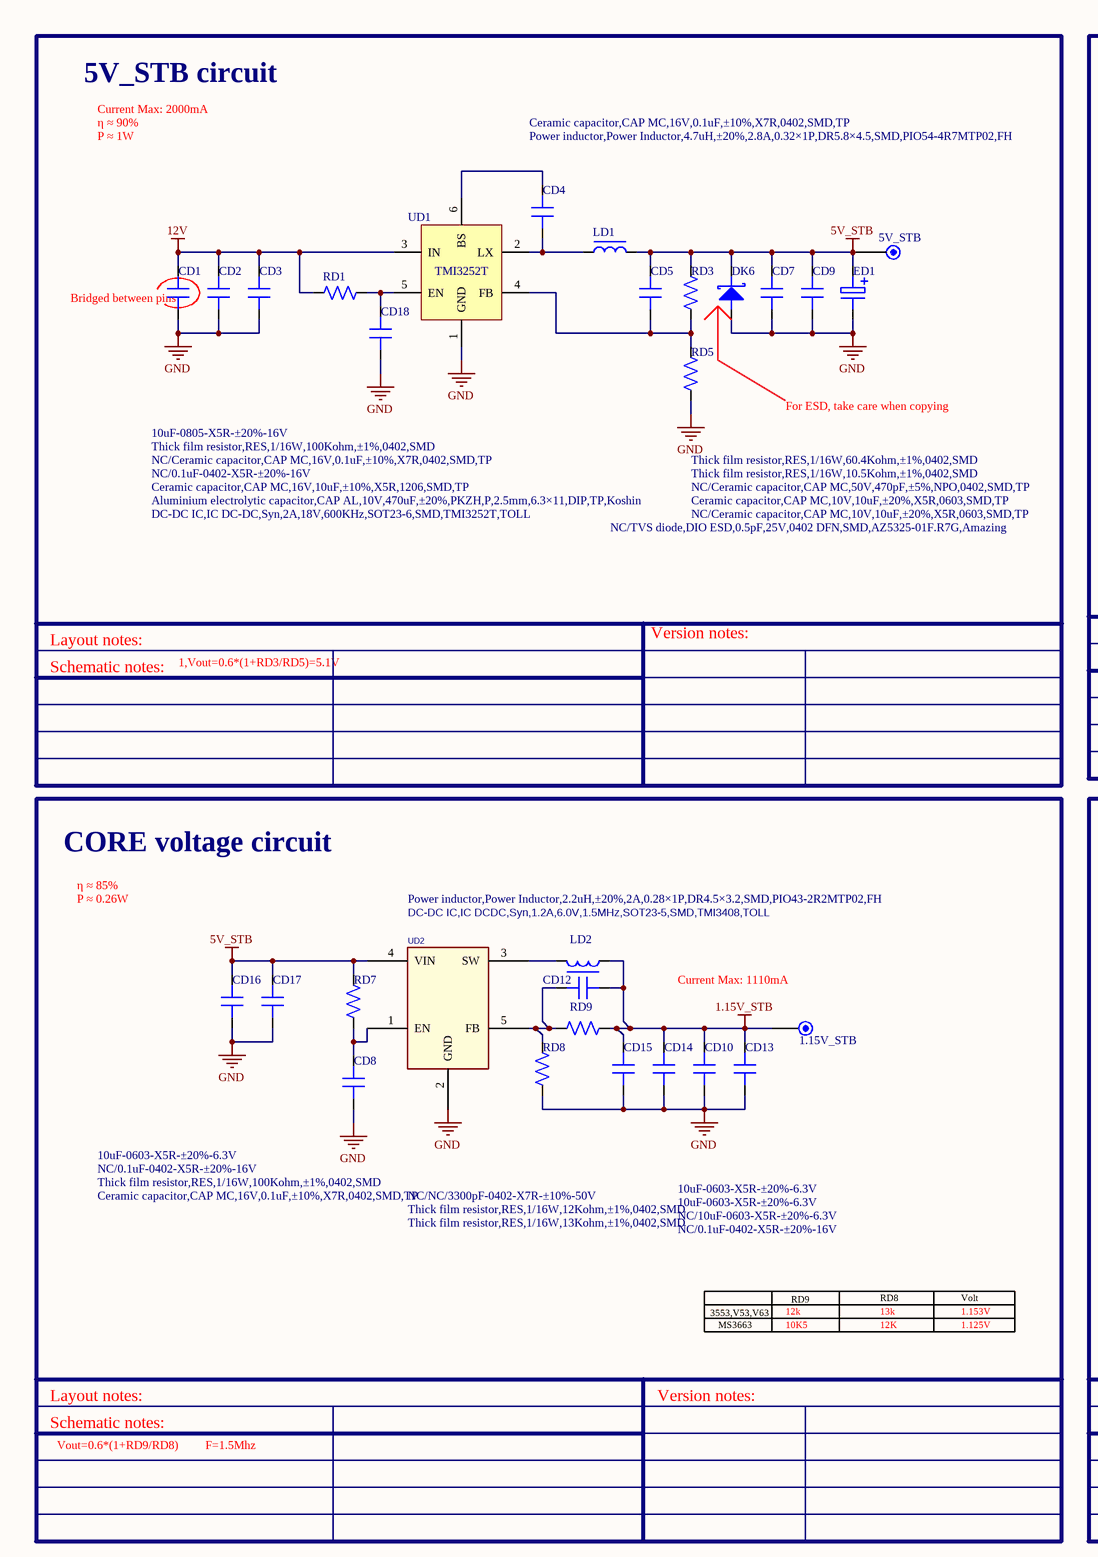
[diagram p0: MISC86383-11.SchDoc, left]
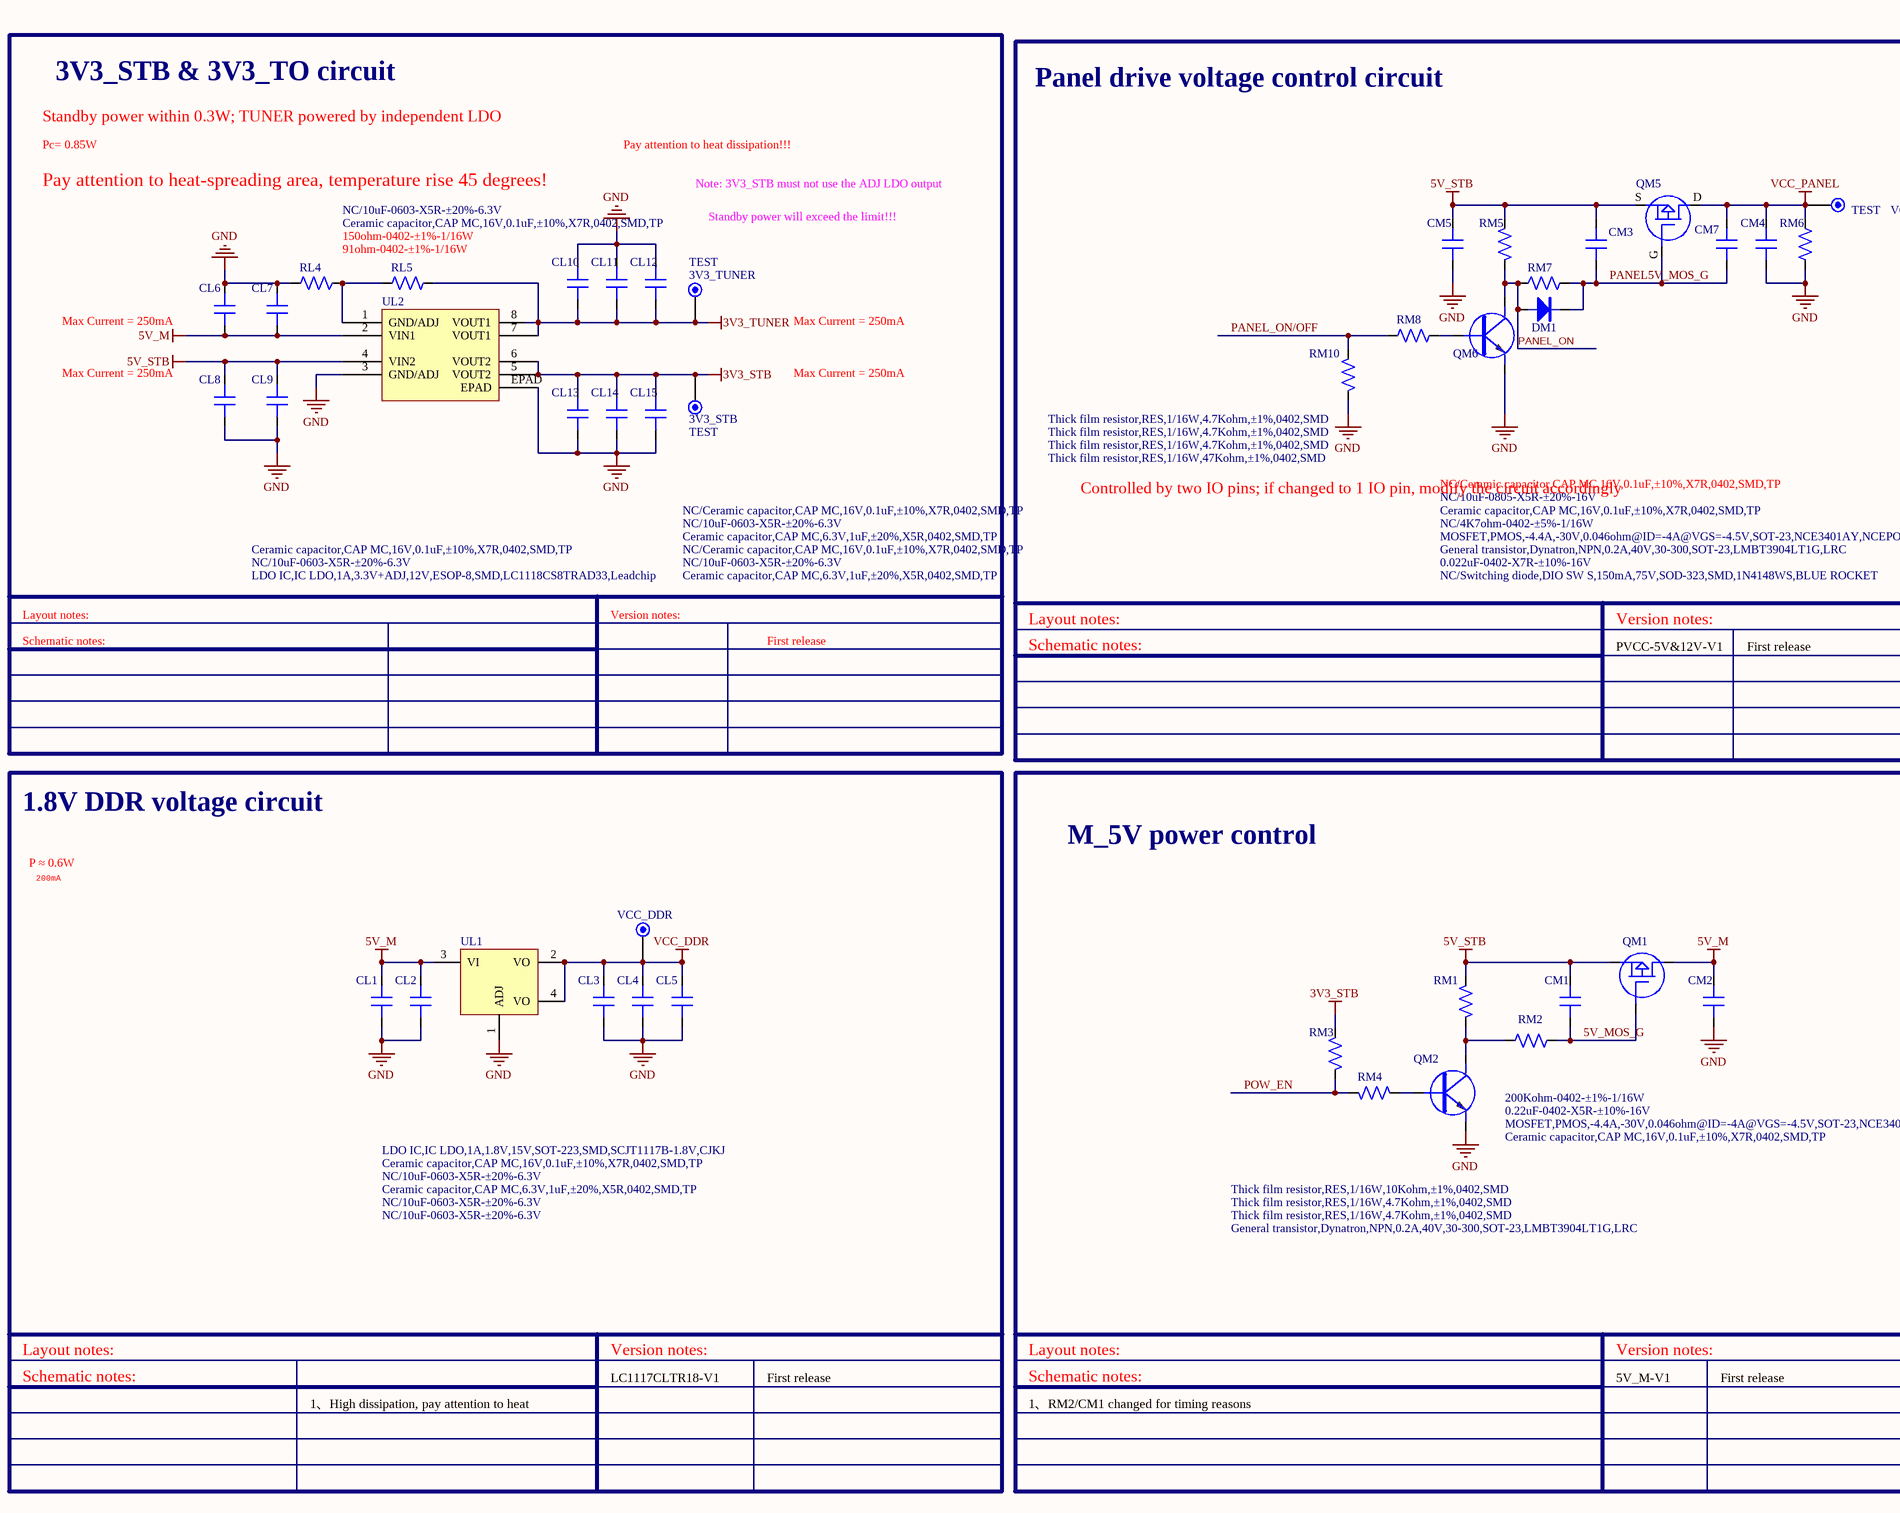
[diagram p1: MISC86383-11.SchDoc, middle]
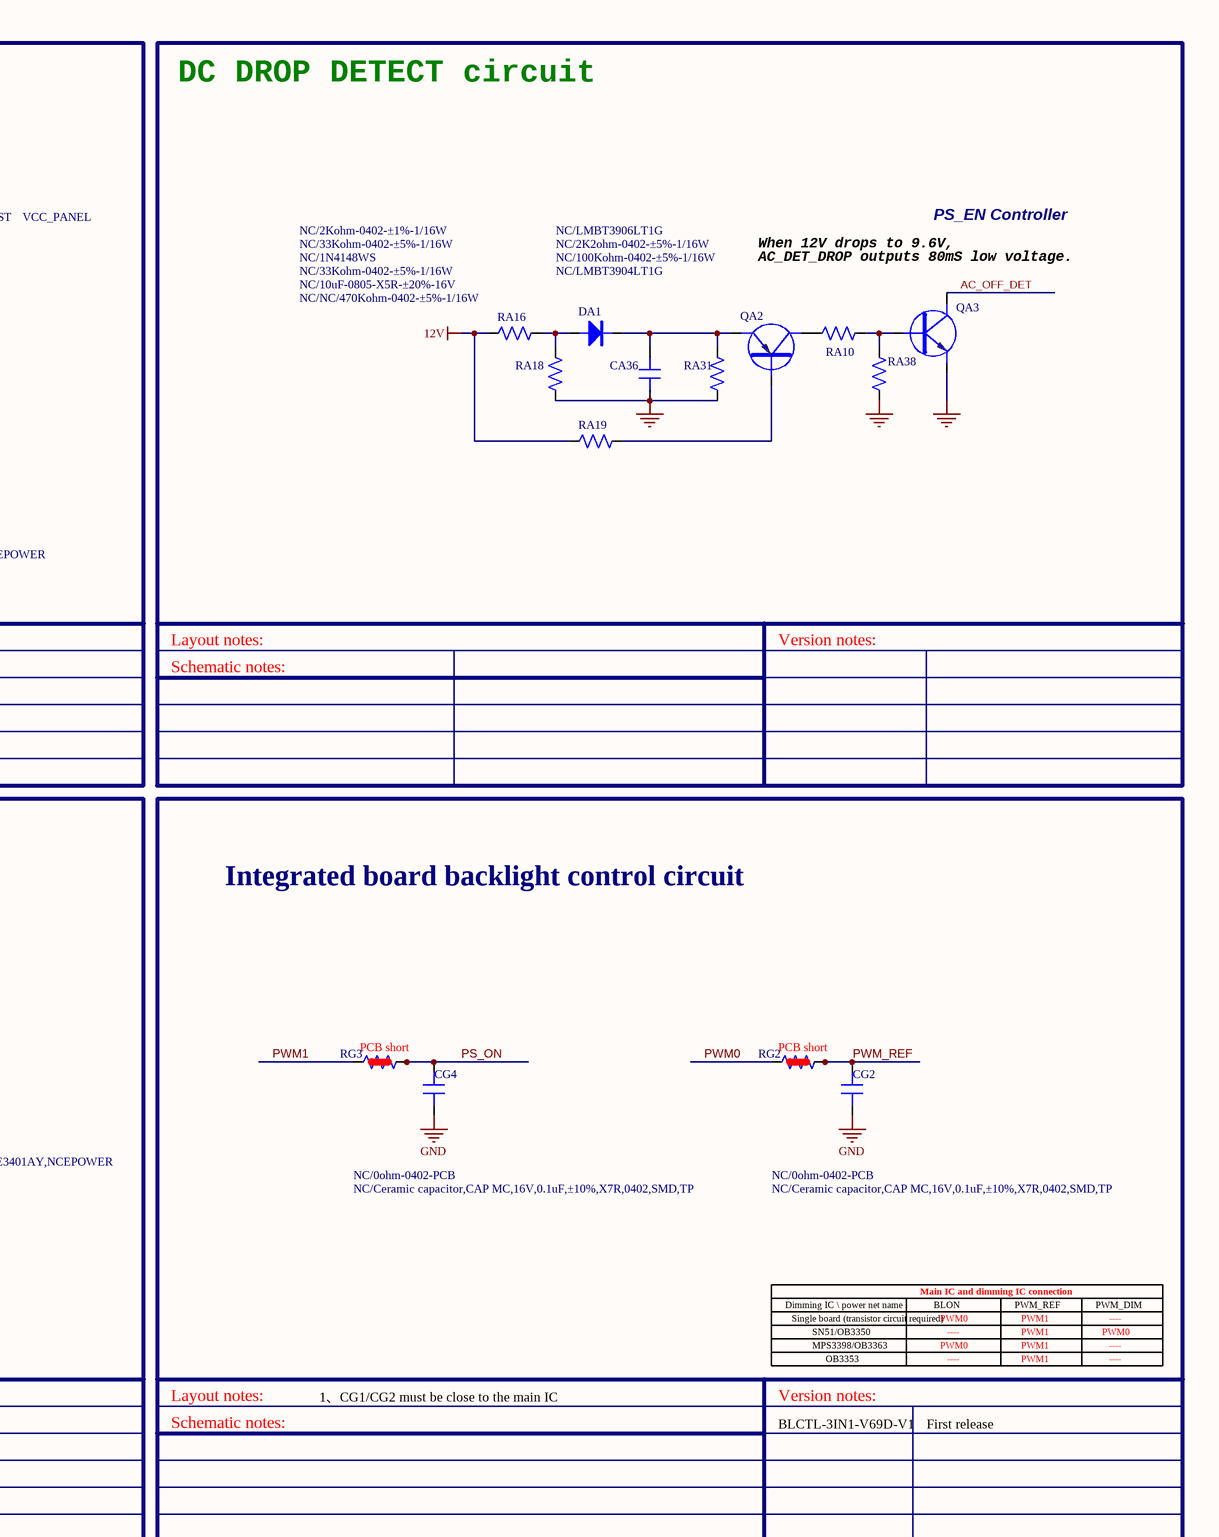
[diagram p2: MISC86383-11.SchDoc, right]
# Altium project MISC86383-33.PrjPCB (part 1 of 8)
9 sheets, 719 parts. Net scope: global (net labels, ports and power ports of the same name join across sheets).
Board files: MISC86383-7.PcbDoc, MISC86383.PcbDoc, MISC86383-9.PcbDoc
Sheets:
  MISC86383-11.SchDoc
  MISC86383-12.SchDoc
  MISC86383-13.SchDoc
  MISC86383-14.SchDoc
  MISC86383-15.SchDoc
  MISC86383-16.SchDoc
  MISC86383-18.SchDoc
  MISC86383-19.SchDoc
  MISC86383-5.SchDoc

## Sheet MISC86383-11.SchDoc
size 812 x 317 mm

### Parts
1.15V_STB  TEST  [TP]  (value not drawn)
3V3_STB  TEST  [TP]
3V3_TUNER  TEST  [TP]
5V_STB  TEST  [TP]  (value not drawn)
CA36  NC/10uF-0805-X5R-±20%-16V  [C0805]
CD1  Ceramic capacitor,CAP MC,16V,10uF,±10%,X5R,1206,SMD,TP  [C1206]
CD2  10uF-0805-X5R-±20%-16V  [C0805]
CD3  NC/Ceramic capacitor,CAP MC,16V,0.1uF,±10%,X7R,0402,SMD,TP  [C0402]
CD4  Ceramic capacitor,CAP MC,16V,0.1uF,±10%,X7R,0402,SMD,TP  [C0402]
CD5  NC/Ceramic capacitor,CAP MC,50V,470pF,±5%,NPO,0402,SMD,TP  [C0402]
CD7  Ceramic capacitor,CAP MC,10V,10uF,±20%,X5R,0603,SMD,TP  [C0603]
CD8  Ceramic capacitor,CAP MC,16V,0.1uF,±10%,X7R,0402,SMD,TP  [C0402]
CD9  NC/Ceramic capacitor,CAP MC,10V,10uF,±20%,X5R,0603,SMD,TP  [C0603]
CD10  NC/10uF-0603-X5R-±20%-6.3V  [C0603]
CD12  NC/NC/3300pF-0402-X7R-±10%-50V  [C0402]
CD13  NC/0.1uF-0402-X5R-±20%-16V  [C0402]
CD14  10uF-0603-X5R-±20%-6.3V  [C0603]
CD15  10uF-0603-X5R-±20%-6.3V  [C0603]
CD16  10uF-0603-X5R-±20%-6.3V  [C0603]
CD17  NC/0.1uF-0402-X5R-±20%-16V  [C0402]
CD18  NC/0.1uF-0402-X5R-±20%-16V  [C0402]
CG2  NC/Ceramic capacitor,CAP MC,16V,0.1uF,±10%,X7R,0402,SMD,TP  [C0402]
CG4  NC/Ceramic capacitor,CAP MC,16V,0.1uF,±10%,X7R,0402,SMD,TP  [C0402]
CL1  NC/10uF-0603-X5R-±20%-6.3V  [C0603]
CL2  Ceramic capacitor,CAP MC,16V,0.1uF,±10%,X7R,0402,SMD,TP  [C0402]
CL3  Ceramic capacitor,CAP MC,6.3V,1uF,±20%,X5R,0402,SMD,TP  [C0402]
CL4  NC/10uF-0603-X5R-±20%-6.3V  [C0603]
CL5  NC/10uF-0603-X5R-±20%-6.3V  [C0603]
CL6  Ceramic capacitor,CAP MC,16V,0.1uF,±10%,X7R,0402,SMD,TP  [C0402]
CL7  NC/10uF-0603-X5R-±20%-6.3V  [C0603]
CL8  NC/10uF-0603-X5R-±20%-6.3V  [C0603]
CL9  Ceramic capacitor,CAP MC,16V,0.1uF,±10%,X7R,0402,SMD,TP  [C0402]
CL10  NC/Ceramic capacitor,CAP MC,16V,0.1uF,±10%,X7R,0402,SMD,TP  [C0402]
CL11  NC/10uF-0603-X5R-±20%-6.3V  [C0603]
CL12  Ceramic capacitor,CAP MC,6.3V,1uF,±20%,X5R,0402,SMD,TP  [C0402]
CL13  NC/Ceramic capacitor,CAP MC,16V,0.1uF,±10%,X7R,0402,SMD,TP  [C0402]
CL14  NC/10uF-0603-X5R-±20%-6.3V  [C0603]
CL15  Ceramic capacitor,CAP MC,6.3V,1uF,±20%,X5R,0402,SMD,TP  [C0402]
CM1  0.22uF-0402-X5R-±10%-16V  [C0402]
CM2  Ceramic capacitor,CAP MC,16V,0.1uF,±10%,X7R,0402,SMD,TP  [C0402]
CM3  NC/Ceramic capacitor,CAP MC,16V,0.1uF,±10%,X7R,0402,SMD,TP  [C0402]
CM4  Ceramic capacitor,CAP MC,16V,0.1uF,±10%,X7R,0402,SMD,TP  [C0402]
CM5  NC/10uF-0805-X5R-±20%-16V  [C0805]
CM7  0.022uF-0402-X7R-±10%-16V  [C0402]
DA1  NC/1N4148WS  [DIODE-S-12]
DK6  NC/TVS diode,DIO ESD,0.5pF,25V,0402 DFN,SMD,AZ5325-01F.R7G,Amazing  [DIODE-S0402]
DM1  NC/Switching diode,DIO SW S,150mA,75V,SOD-323,SMD,1N4148WS,BLUE ROCKET  [DIODE-S-12]
ED1  Aluminium electrolytic capacitor,CAP AL,10V,470uF,±20%,PKZH,P,2.5mm,6.3×11,DIP,TP,Koshin  [EC(6.3*11)-V-2.5]
LD1  Power inductor,Power Inductor,4.7uH,±20%,2.8A,0.32×1P,DR5.8×4.5,SMD,PIO54-4R7MTP02,FH  [L(5.8*4.5)-S]
LD2  Power inductor,Power Inductor,2.2uH,±20%,2A,0.28×1P,DR4.5×3.2,SMD,PIO43-2R2MTP02,FH  [L(4.5*3.5)-S]
QA2  NC/LMBT3906LT1G  [SOT-23]
QA3  NC/LMBT3904LT1G  [SOT-23]
QM1  MOSFET,PMOS,-4.4A,-30V,0.046ohm@ID=-4A@VGS=-4.5V,SOT-23,NCE3401AY,NCEPOWER  [SOT-23-1]
QM2  General transistor,Dynatron,NPN,0.2A,40V,30-300,SOT-23,LMBT3904LT1G,LRC  [SOT-23]
QM5  MOSFET,PMOS,-4.4A,-30V,0.046ohm@ID=-4A@VGS=-4.5V,SOT-23,NCE3401AY,NCEPOWER  [SOT-23-1]
QM6  General transistor,Dynatron,NPN,0.2A,40V,30-300,SOT-23,LMBT3904LT1G,LRC  [SOT-23]
RA10  NC/2K2ohm-0402-±5%-1/16W  [R0402]
RA16  NC/2Kohm-0402-±1%-1/16W  [R0402]
RA18  NC/33Kohm-0402-±5%-1/16W  [R0402]
RA19  NC/33Kohm-0402-±5%-1/16W  [R0402]
RA31  NC/NC/470Kohm-0402-±5%-1/16W  [R0402]
RA38  NC/100Kohm-0402-±5%-1/16W  [R0402]
RD1  Thick film resistor,RES,1/16W,100Kohm,±1%,0402,SMD  [R0402]
RD3  Thick film resistor,RES,1/16W,60.4Kohm,±1%,0402,SMD  [R0402]
RD5  Thick film resistor,RES,1/16W,10.5Kohm,±1%,0402,SMD  [R0402]
RD7  Thick film resistor,RES,1/16W,100Kohm,±1%,0402,SMD  [R0402]
RD8  Thick film resistor,RES,1/16W,13Kohm,±1%,0402,SMD  [R0402]
RD9  Thick film resistor,RES,1/16W,12Kohm,±1%,0402,SMD  [R0402]
RG2  NC/0ohm-0402-PCB  [R0402SC]
RG3  NC/0ohm-0402-PCB  [R0402SC]
RL4  150ohm-0402-±1%-1/16W  [R0402]
RL5  91ohm-0402-±1%-1/16W  [R0402]
RM1  Thick film resistor,RES,1/16W,4.7Kohm,±1%,0402,SMD  [R0402]
RM2  200Kohm-0402-±1%-1/16W  [R0402]
RM3  Thick film resistor,RES,1/16W,10Kohm,±1%,0402,SMD  [R0402]
RM4  Thick film resistor,RES,1/16W,4.7Kohm,±1%,0402,SMD  [R0402]
RM5  Thick film resistor,RES,1/16W,4.7Kohm,±1%,0402,SMD  [R0402]
RM6  NC/4K7ohm-0402-±5%-1/16W  [R0402]
RM7  Thick film resistor,RES,1/16W,47Kohm,±1%,0402,SMD  [R0402]
RM8  Thick film resistor,RES,1/16W,4.7Kohm,±1%,0402,SMD  [R0402]
RM10  Thick film resistor,RES,1/16W,4.7Kohm,±1%,0402,SMD  [R0402]
UD1  DC-DC IC,IC DC-DC,Syn,2A,18V,600KHz,SOT23-6,SMD,TMI3252T,TOLL  [TSOT23-6]
UD2  DC-DC IC,IC DCDC,Syn,1.2A,6.0V,1.5MHz,SOT23-5,SMD,TMI3408,TOLL  [SOT-23-5]
UL1  LDO IC,IC LDO,1A,1.8V,15V,SOT-223,SMD,SCJT1117B-1.8V,CJKJ  [SOT-223]
UL2  LDO IC,IC LDO,1A,3.3V+ADJ,12V,ESOP-8,SMD,LC1118CS8TRAD33,Leadchip  [SOP8/1.27-3]
VCC_DDR  TEST  [TP]  (value not drawn)
VCC_PANEL  TEST  [TP]

### Blocks framed on the sheet
5V_STB circuit: 5V_STB CD1-CD5 CD7 CD9 CD18 DK6 ED1 LD1 RD1 RD3 RD5 UD1
3V3_STB & 3V3_TO circuit: 3V3_STB 3V3_TUNER CL6-CL15 RL4 RL5 UL2
Panel drive voltage control circuit: CM3-CM5 CM7 DM1 QM5 QM6 RM5-RM8 RM10 VCC_PANEL
DC DROP DETECT circuit: CA36 DA1 QA2 QA3 RA10 RA16 RA18 RA19 RA31 RA38
CORE voltage circuit: 1.15V_STB CD8 CD10 CD12-CD17 LD2 RD7-RD9 UD2
1.8V DDR voltage circuit: CL1-CL5 UL1 VCC_DDR
M_5V power control: CM1 CM2 QM1 QM2 RM1-RM4
Integrated board backlight control circuit: CG2 CG4 RG2 RG3

### Nets
1.15V_STB: 1.15V_STB.1 CD10.2 CD12.2 CD13.2 CD14.2 CD15.2 LD2.1 RD9.1
3V3_STB: 3V3_STB.1 CL13.1 CL14.1 CL15.1 RM3.1 UL2.5(VOUT2) UL2.6(VOUT2)
3V3_TUNER: 3V3_TUNER.1 CL10.2 CL11.1 CL12.2 RL5.2 UL2.7(VOUT1) UL2.8(VOUT1)
5V_M: CL1.2 CL2.2 CL6.2 CL7.2 CM2.1 QM1.D UL1.3(VI) UL2.2(VIN1)
5V_STB: 5V_STB.1 CD5.2 CD7.2 CD9.2 CD16.2 CD17.2 CL8.2 CL9.2 CM1.1 CM3.2 CM5.2 DK6.K ED1.1 LD1.2 QM1.S QM5.S RD3.2 RD7.2 RM1.2 RM5.2 UD2.4(VIN) UL2.4(VIN2)
12V: CD1.2 CD2.1 CD3.2 RA16.1 RA19.2 RD1.1 UD1.3(IN)
GND: CA36.1 CD1.1 CD2.2 CD3.1 CD7.1 CD8.1 CD9.1 CD10.1 CD13.1 CD14.1 CD15.1 CD16.1 CD17.1 CD18.1 CG2.2 CG4.2 CL1.1 CL2.1 CL3.1 CL4.1 CL5.1 CL6.1 CL7.1 CL8.1 CL9.1 CL10.1 CL11.2 CL12.1 CL13.2 CL14.2 CL15.2 CM2.2 CM4.2 CM5.1 DK6.A ED1.2 QA3.E QM2.E QM6.E RA18.1 RA31.1 RA38.1 RD5.1 RD8.2 RL4.1 RM6.2 RM10.2 UD1.1(GND) UD2.2(GND) UL1.1(ADJ) UL2.3(GND/ADJ) UL2.EPAD
PS_ON: CG4.1 RG3.2 RG3.3
PWM_REF: CG2.1 RG2.2 RG2.3
VCC_DDR: CL3.2 CL4.2 CL5.2 UL1.2(VO) UL1.4(VO) VCC_DDR.1
VCC_PANEL: CM4.1 CM7.2 QM5.D RM6.1 VCC_PANEL.1
5V_MOS_G: CM1.2 QM1.G RM2.2
AC_OFF_DET: QA3.C
PANEL5V_MOS_G: CM3.1 CM7.1 DM1.K QM5.G RM7.2
PANEL_ON: DM1.A QM6.C RM5.1 RM7.1
PANEL_ON/OFF: RM8.1 RM10.1
POW_EN: RM3.2 RM4.2
PWM0: RG2.1
PWM1: RG3.1
NetCA36_2: CA36.2 DA1.K QA2.E RA31.2
NetCD4_1: CD4.1 LD1.1 UD1.2(LX)
NetCD4_2: CD4.2 UD1.6(BS)
NetCD5_1: CD5.1 RD3.1 RD5.2 UD1.4(FB)
NetCD8_2: CD8.2 RD7.1 UD2.1(EN)
NetCD12_1: CD12.1 RD8.1 RD9.2 UD2.5(FB)
NetCD18_2: CD18.2 RD1.2 UD1.5(EN)
NetDA1_A: DA1.A RA16.2 RA18.2
NetLD2_2: LD2.2 UD2.3(SW)
NetQA2_B: QA2.B RA19.1
NetQA2_C: QA2.C RA10.1
NetQA3_B: QA3.B RA10.2 RA38.2
NetQM2_B: QM2.B RM4.1
NetQM2_C: QM2.C RM1.1 RM2.1
NetQM6_B: QM6.B RM8.2
NetRL4_2: RL4.2 RL5.1 UL2.1(GND/ADJ)

### Notes on the sheet
- Current Max: 2000mA
- η ≈ 90%
- P ≈ 1W
- Standby power within 0.3W; TUNER powered by independent LDO
- Pc= 0.85W
- Pay attention to heat dissipation!!!
- Pay attention to heat-spreading area, temperature rise 45 degrees!
- Note: 3V3_STB must not use the ADJ LDO output
- Standby power will exceed the limit!!!
- When 12V drops to 9.6V,
- PS_EN Controller
- (near CD1) Bridged between pins
- (near QA3) AC_DET_DROP outputs 80mS low voltage.
- Max Current = 250mA
- For ESD, take care when copying
- Controlled by two IO pins; if changed to 1 IO pin, modify the circuit accordingly
- Layout notes:
- Version notes:
- Schematic notes:
- 1,Vout=0.6*(1+RD3/RD5)=5.1V
- First release
- PVCC-5V&12V-V1
- η ≈ 85%
- P ≈ 0.26W
- P ≈ 0.6W
- 200mA
- Current Max: 1110mA
- 3553,V53,V63
- MS3663
- 12k
- 10K5
- RD9
- RD8
- 13k
- 12K
- Volt
- 1.153V
- 1.125V
- Dimming IC \ power net name
- Single board (transistor circuit required)
- Main IC and dimming IC connection
- BLON
- PWM0
- PWM_REF
- PWM1
- PWM_DIM
- ----
- 1、CG1/CG2 must be close to the main IC
- SN51/OB3350
- MPS3398/OB3363
- OB3353
- Vout=0.6*(1+RD9/RD8)
- F=1.5Mhz
- 1、High dissipation, pay attention to heat
- LC1117CLTR18-V1
- 1、RM2/CM1 changed for timing reasons
- 5V_M-V1
- BLCTL-3IN1-V69D-V1

### Library data of the parts
CA36 CM5 = 10uF-0805-X5R-±20%-16V-D
CD1 = 004.003.0000514-D: Ceramic capacitor,CAP MC,16V,10uF,±10%,X5R,1206,SMD,TP-D
CD2 = 004.003.0000386-D: Ceramic capacitor,CAP MC,16V,10uF,±20%,X5R,0805,SMD,TP-D
CD3 CD4 CD8 CD18 = 004.003.0000403-D: Ceramic capacitor,CAP MC,16V,0.1uF,±20%,X5R,0402,SMD,TP-D
CD5 = 004.003.0000558-D: Ceramic capacitor,CAP MC,50V,470pF,±5%,NPO,0402,SMD,TP-D
CD7 CD9 = 004.003.0000394-D: Ceramic capacitor,CAP MC,10V,10uF,±20%,X5R,0603,SMD,TP-D
CD10 CD14-CD16 CL1 CL4 CL5 CL7 CL8 CL11 CL14 = 10uF-0603-X5R-±20%-6.3V-D
CD12 = 3300pF-0402-X7R-±10%-50V-D
CD13 CD17 CL6 CL9 CL10 CL12 CL13 CL15 CM3 = 0.1uF-0402-X5R-±20%-16V-D
CG2 CG4 CL2 CL3 CM1 CM2 CM4 = 0.1uF-0402-Y5V-+80%-20%-16V-D
CM7 = 0.022uF-0402-X7R-±10%-16V-D
DA1 DM1 = 1N4148WS-D
DK6 = 004.005.0000435: TVS diode,DIO ESD,0.5pF,25V,0402 DFN,SMD,AZ5325-01F.R7G,Amazing-D
ED1 = 470uF-10V-±20%-6.3×11-105℃-黑底白字-编带-F=2.5-XF-DHAI: Electrolytic
LD1 = 004.004.0000017-D: Power inductor,Power Inductor,4.7uH,±20%,2.8A,0.35×1P,DR5.8×4.5,SMD,SCD54TL-4R7M,Soldier-D
LD2 = SLN43T-6R8M-D
QA2 = 3CG3906M-D: Q-PNP-#-#-#
QA3 = MMBT3904(f≥350MHz)-D-NPN: Q-NPN-#-#-#
QM1 = WPM2341A-3/TR-D
QM2 QM6 = LMBT3904LT1G-D-NPN: Q-NPN-#-#-#
QM5 = WPM3407C-3/TR-D
RA10 = 1Kohm-0402-±5%-1/16W-D
RA16 = 8K2ohm-0402-±5%-1/16W-D
RA18 RA19 = 33Kohm-0402-±5%-1/16W-D
RA31 = 470Kohm-0402-±5%-1/16W-D
RA38 RM2 = 100Kohm-0402-±5%-1/16W-D
RD1 RD7 = 004.002.0000579-D: Thick film resistor,RES,1/16W,100Kohm,±5%,0402,SMD-D
RD3 = 004.002.0000806-D: Thick film resistor,RES,1/16W,60.4Kohm,±1%,0402,SMD-D
RD5 = 004.002.0000573-D: Thick film resistor,RES,1/16W,10.5Kohm,±1%,0402,SMD-D
RD8 = 004.002.0000593-D: Thick film resistor,RES,1/16W,13Kohm,±1%,0402,SMD-D
RD9 = 004.002.0000588-D: Thick film resistor,RES,1/16W,12Kohm,±1%,0402,SMD-D
RG2 RG3 = 0ohm-0402-PCB-D
RL4 = 150ohm-0402-±1%-1/16W-D
RL5 = 91ohm-0402-±1%-1/16W-D
RM1 RM5 RM6 RM8 = 4k7ohm-0402-±5%-1/16W-D
RM3 RM4 = 10Kohm-0402-±5%-1/16W-D
RM7 = 47Kohm-0402-±5%-1/16W-D
RM10 = 2K2ohm-0402-±5%-1/16W-D
UD1 = 004.010.0001184-D: DC-DC IC,IC DC-DC,Syn,2A,18V,600KHz,SOT23-6,SMD,TMI3252T,TOLL-D
UD2 = DC-DC芯片,IC DCDC,Syn,1.2A,7.0V,1.5MHz,SOT23-5,SMD,LC2127CB5TR,Leadchip-D
UL1 = LC1117CLTR18-D
UL2 = LC1118-D